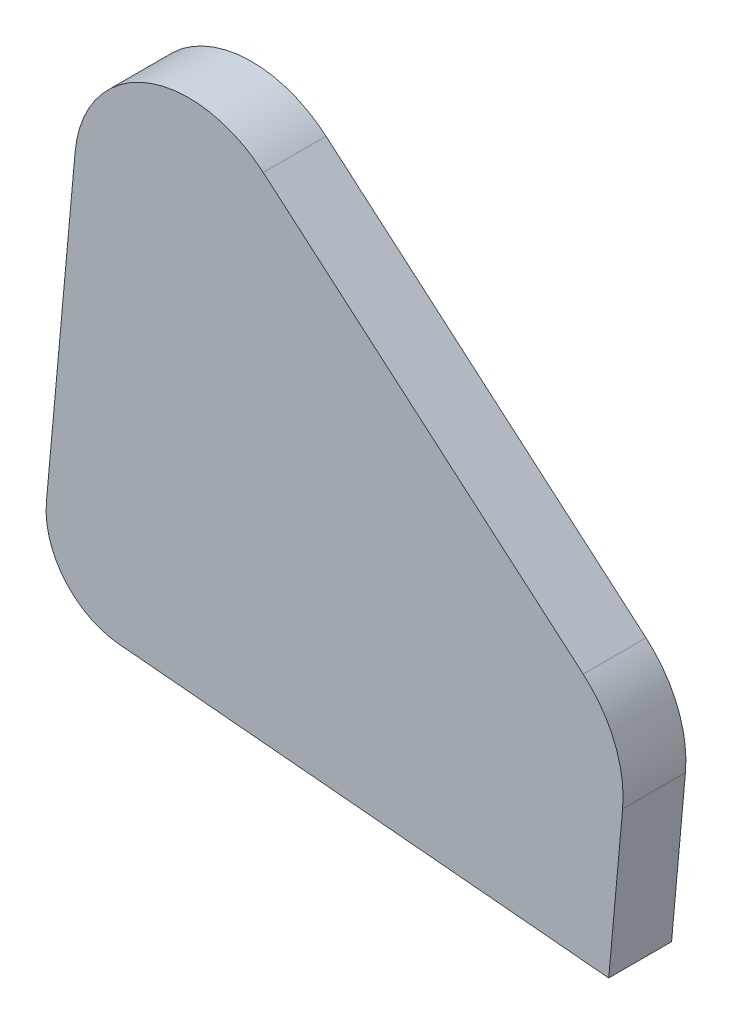
from build123d import *

# Parameters (mm, degrees)
BOSS_EXTRUDE2_DEPTH = 110
SHELL2_T            = -3


with BuildPart() as part:
    # Sketch1 → Boss-Extrude2 (new body)
    with BuildSketch(Plane.XY):
        with BuildLine():
            Line((-199.186622288, 18.019142639), (-249.430635602, -537.386600152))
            ThreePointArc((-249.430635602, -537.386600152), (-217.511368505, -639.673327373), (-122.613399848, -689.430635602))
            Line((-122.613399848, -689.430635602), (735.059712531, -767.018848969))
            Line((735.059712531, -767.018848969), (759.356160444, -498.441842272))
            ThreePointArc((759.356160444, -498.441842272), (745.466568798, -405.15643604), (690.371143367, -328.608530331))
            Line((690.371143367, -328.608530331), (130.201605211, 151.814169301))
            ThreePointArc((130.201605211, 151.814169301), (-75.266263592, 185.297030642), (-199.186622288, 18.019142639))
        make_face()
    extrude(amount=BOSS_EXTRUDE2_DEPTH)

    # Shell2
    shell2_openings = [part.faces().sort_by_distance(p)[0] for p in [
        (206.21225605, -348.127169203, 0),
    ]]
    offset(amount=SHELL2_T, openings=shell2_openings, kind=Kind.INTERSECTION)


solid = part.part
